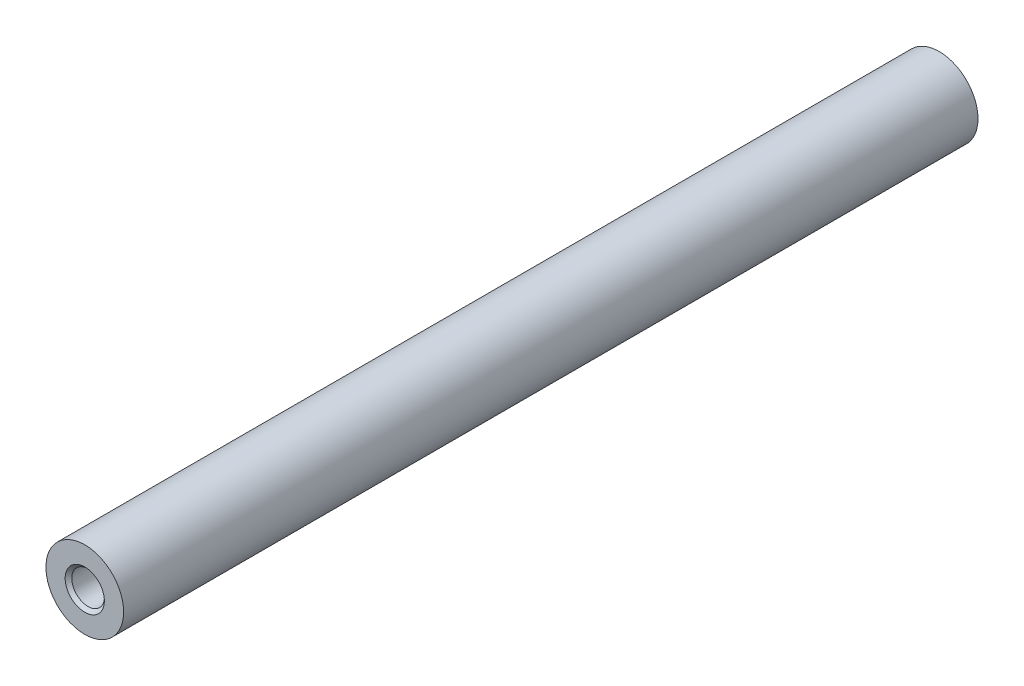
SolidWorks part; units mm, degrees
ref_plane "前视基准面" through (0, 0, 0) normal (0, 0, 1) x (1, 0, 0)
ref_plane "上视基准面" through (0, 0, 0) normal (0, 1, 0) x (1, 0, 0)
ref_plane "右视基准面" through (0, 0, 0) normal (1, 0, 0) x (0, 0, -1)
sketch "草图1" plane through (0, 0, 0) normal (0, 0, 1) x (1, 0, 0)
  circle A0 centre (0, 0) radius 5
  dimension "D1" = 10
extrude "凸台-拉伸1" add sketch "草图1" along normal mid plane 110
sketch "草图2" plane through (0, 0, 55) normal (0, 0, 1) x (1, 0, 0)
  circle A0 centre (0, 0) radius 0.295
hole_wizard "M5x0.8 螺纹孔1" positions "3D草图1" profile "草图3" tap size "M5x0.8" standard "BSI"
sketch3d "3D草图1"
  point P3 (0, 0, 55)
sketch "草图3" plane through (0, 0, 55) normal (1, 0, 0) x (0, -1, 0)
  line L0 (0, 0) -> (0, 13.6618)
  line L1 (0, 13.6618) -> (2.1, 12.4)
  line L2 (2.1, 12.4) -> (2.1, 0.425)
  line L3 (2.1, 0.425) -> (2.525, 0)
  line L5 (2.525, 0) -> (0, 0)
  line L6 (-2.1, 0.425) -> (-2.525, 0) construction
  line L10 (0, 13.6618) -> (-2.1, 12.4) construction
  line L11 (0, -6.35) -> (0, 107.95) construction
  dimension "螺纹孔钻头直径" = 4.2
  dimension "螺纹孔钻头深度" = 12.4
  dimension "近端锥形沉头孔直径" = 5.05
  dimension "近端锥形沉头孔角度" = 90
  dimension "导头角度" = 118
cosmetic thread "孔螺蚊线1"
mirror "镜向1" about plane through (0, 0, 0) normal (0, 0, 1) of "M5x0.8 螺纹孔1"
cosmetic thread "孔螺蚊线2" parameters "D1"=10, "D2"=5
